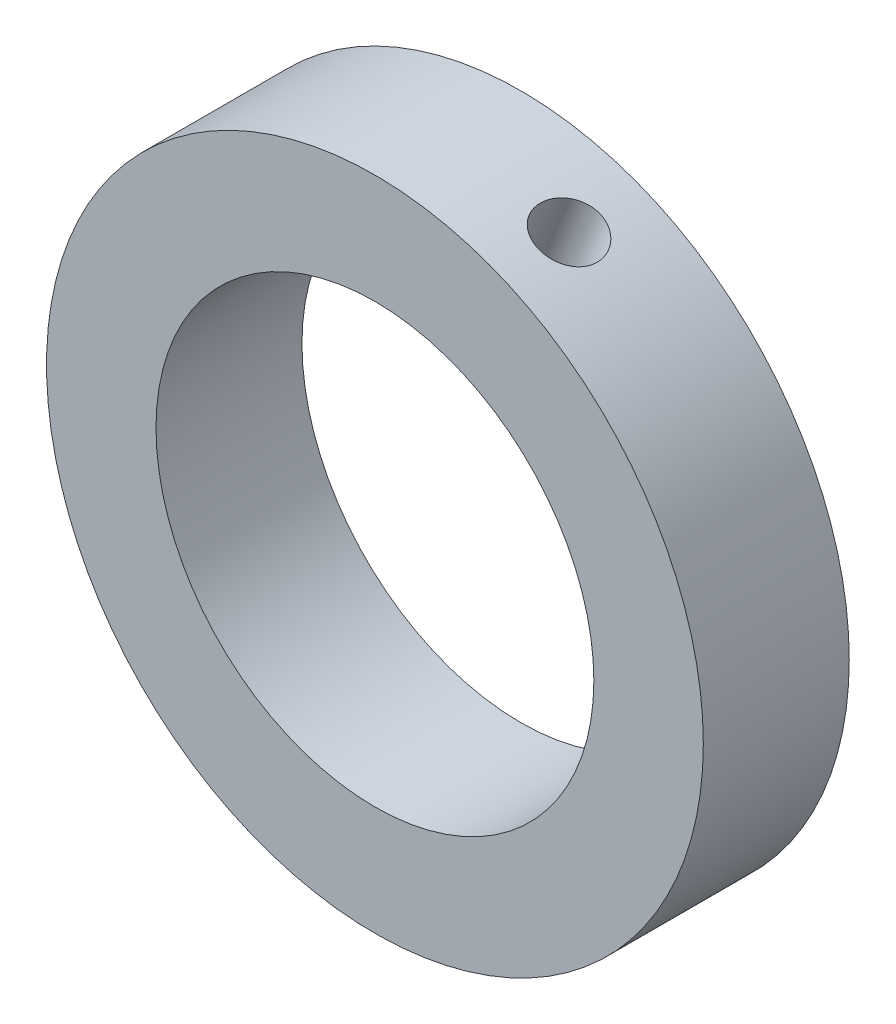
from build123d import *

# Parameters (mm, degrees)
SKETCH1_R              = 22.5
SKETCH1_R_2            = 15
BOSS_EXTRUDE1_DEPTH    = 10
M5_TAPPED_HOLE1_REACH  = 55.492
M5_TAPPED_HOLE1_BORE_R = 2.1


with BuildPart() as part:
    # Sketch1 → Boss-Extrude1 (new body)
    with BuildSketch(Plane.XY):
        Circle(SKETCH1_R)
        Circle(SKETCH1_R_2, mode=Mode.SUBTRACT)
    extrude(amount=BOSS_EXTRUDE1_DEPTH)

    # M5 Tapped Hole1 bore (on position points) → M5 Tapped Hole1 (cut, up to next)
    with BuildSketch(Plane(origin=(8.385619335, 20.878970002, 5.06911991), x_dir=(0.927954222329, -0.372694192686, 0), z_dir=(0.372694192686, 0.927954222329, 0)), mode=Mode.PRIVATE) as m5_tapped_hole1_sk1:
        Circle(M5_TAPPED_HOLE1_BORE_R)
    m5_tapped_hole1_tool1 = extrude(m5_tapped_hole1_sk1.sketch, amount=-M5_TAPPED_HOLE1_REACH, mode=Mode.PRIVATE) & part.part
    add(m5_tapped_hole1_tool1.solids().sort_by_distance((8.385619, 20.87897, 5.06912))[0], mode=Mode.SUBTRACT)


solid = part.part
